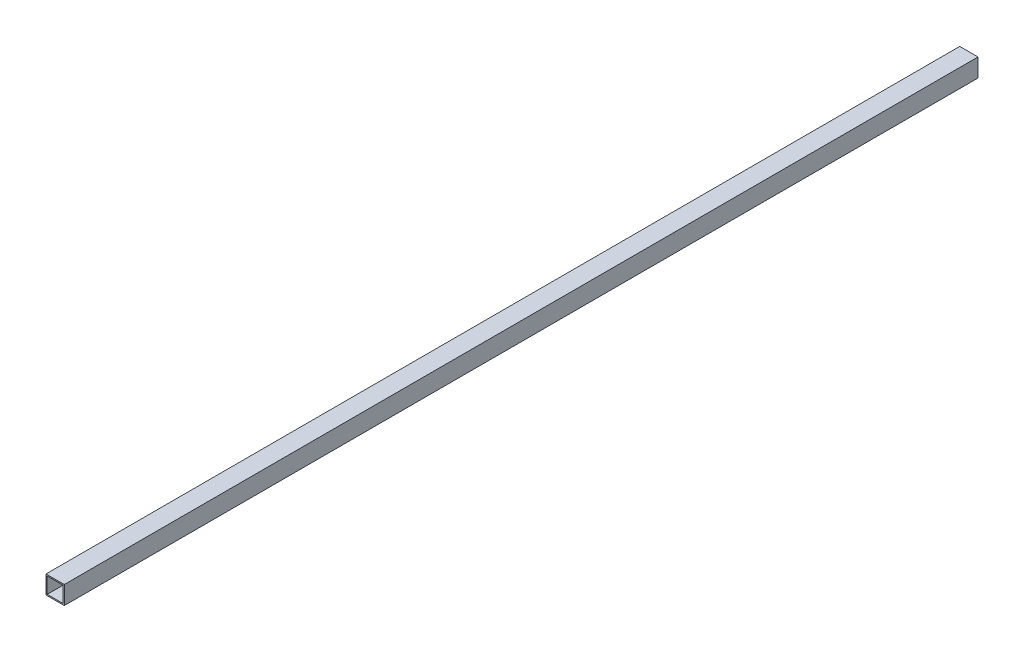
SolidWorks part; units mm, degrees
ref_plane "前视基准面" through (0, 0, 0) normal (0, 0, 1) x (1, 0, 0)
ref_plane "上视基准面" through (0, 0, 0) normal (0, 1, 0) x (1, 0, 0)
ref_plane "右视基准面" through (0, 0, 0) normal (1, 0, 0) x (0, 0, -1)
sketch "草图1" plane through (0, 0, 0) normal (0, 0, 1) x (1, 0, 0)
  line L0 (13, 13) -> (-13, 13)
  line L1 (15, -15) -> (-15, -15)
  line L2 (15, -15) -> (15, 15)
  line L3 (15, 15) -> (-15, 15)
  line L4 (-15, -15) -> (-15, 15)
  line L5 (15, -15) -> (-15, 15) construction
  line L6 (15, 15) -> (-15, -15) construction
  line L7 (-13, -13) -> (-13, 13)
  line L8 (13, -13) -> (-13, -13)
  line L9 (13, -13) -> (13, 13)
  point P0 (0, 0)
  dimension "D1" = 30
  dimension "D2" = 2
extrude "凸台-拉伸1" add sketch "草图1" along normal mid plane 1500
sketch "草图2" plane through (0, 0, 750) normal (0, 0, 1) x (1, 0, 0)
  circle A1 centre (0, 0) radius 13.1935
